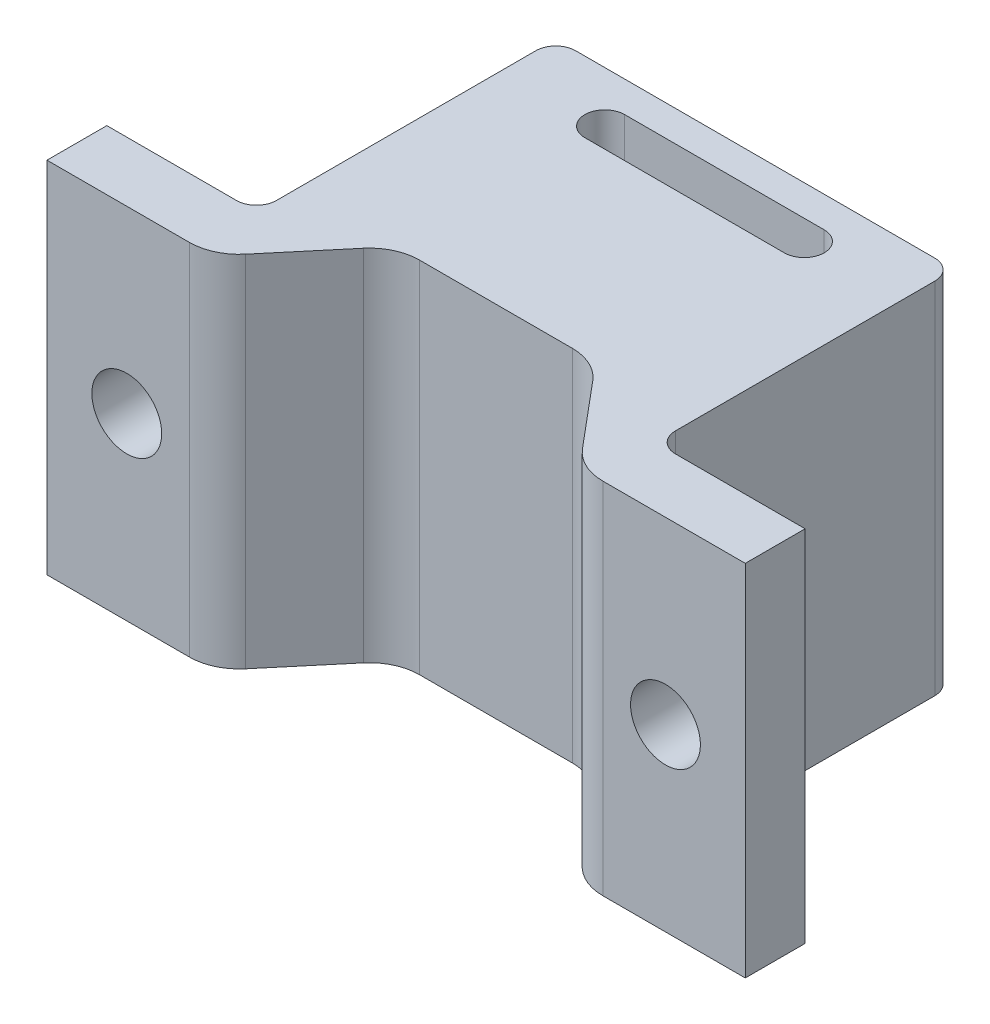
SolidWorks part; units mm, degrees
ref_plane "Front" through (0, 0, 0) normal (0, 0, 1) x (1, 0, 0)
ref_plane "Top" through (0, 0, 0) normal (0, 1, 0) x (1, 0, 0)
ref_plane "Right" through (0, 0, 0) normal (1, 0, 0) x (0, 0, -1)
sketch "Sketch1" plane through (0, 0, 0) normal (0, 1, 0) x (1, 0, 0)
  line L0 (-20, -13.7446) -> (-20, 16.2554)
  line L3 (-20, 16.2554) -> (20, 16.2554)
  line L5 (20, -13.7446) -> (20, 16.2554)
  line L6 (-18.391, -19.7446) -> (-10, -9.7446)
  line L7 (-35, -19.7446) -> (-18.391, -19.7446)
  line L8 (-35, -19.7446) -> (-35, -13.7446)
  line L9 (-35, -13.7446) -> (-20, -13.7446)
  line L10 (35, -19.7446) -> (35, -13.7446)
  line L11 (-10, -9.7446) -> (10, -9.7446)
  line L12 (10, -9.7446) -> (18.391, -19.7446)
  line L13 (20, -13.7446) -> (35, -13.7446)
  line L14 (18.391, -19.7446) -> (35, -19.7446)
  line L15 (-10, 11.1674) -> (10, 11.1674) construction
  line L16 (-10, 13.1674) -> (10, 13.1674)
  line L17 (-10, 9.1674) -> (10, 9.1674)
  arc A0 (-10, 13.1674) -> (-10, 9.1674) centre (-10, 11.1674) ccw
  arc A1 (10, 9.1674) -> (10, 13.1674) centre (10, 11.1674) ccw
  point P0 (0, 0)
  point P6 (0, -9.7446)
  point P11 (0, 11.1674)
  dimension "D14" = 2
  dimension "D1" = 70
  dimension "D2" = 36
  dimension "D3" = 40
  dimension "D4" = 15
  dimension "D5" = 20
  dimension "D6" = 6
  dimension "D7" = 6
  dimension "D8" = 0
  dimension "D9" = 20
  dimension "D10" = 10
  dimension "D11" = 80
  dimension "D12" = 40
  dimension "D13" = 40
extrude "Boss-Extrude1" add sketch "Sketch1" along normal blind 36
fillet "Fillet1" radius 5 4 edges at (18.391, 18, 19.7446) (10, 18, 9.7446) (-10, 18, 9.7446) (-18.391, 18, 19.7446)
fillet "Fillet2" radius 2 2 edges at (20, 18, 13.7446) (-20, 18, 13.7446)
sketch "Sketch2" plane through (0, 0, 13.7446) normal (0, 0, -1) x (-1, 0, 0)
  circle A0 centre (-27, 18) radius 3.5
  circle A1 centre (27, 18) radius 3.5
  dimension "D1" = 54
  dimension "D2" = 7
  dimension "D3" = 7
  dimension "D4" = 27
extrude "Cut-Extrude1" cut sketch "Sketch2" against normal through all
sketch "Sketch3" plane through (0, 0, -16.2554) normal (0, 0, -1) x (-1, 0, 0)
  line L1 (-20, 0) -> (20, 0) construction
  circle A0 centre (0, 18) radius 10
  dimension "D1" = 20
  dimension "D2" = 18
extrude "Cut-Extrude2" cut sketch "Sketch3" against normal blind 6
sketch "Sketch4" plane through (0, 0, -9.1674) normal (0, 0, -1) x (-1, 0, 0)
  circle A0 centre (0, 18) radius 8
  dimension "D1" = 16
extrude "Boss-Extrude2" add sketch "Sketch4" along normal blind 11.09
hole_wizard "M8 Tapped Hole1" positions "Sketch5" profile "Sketch6" tap size "M8" standard "GB"
sketch "Sketch5" plane through (0, 0, -20.2574) normal (0, 0, -1) x (-1, 0, 0)
  point P0 (0, 18)
sketch "Sketch6" plane through (0, 18, -20.2574) normal (1, 0, 0) x (0, 1, 0)
  line L0 (0, 0) -> (0, 24.2929)
  line L1 (0, 24.2929) -> (3.4, 22.25)
  line L2 (3.4, 22.25) -> (3.4, 0)
  line L5 (3.4, 0) -> (0, 0)
  line L10 (0, 24.2929) -> (-3.4, 22.25) construction
  line L11 (0, -6.35) -> (0, 107.95) construction
  dimension "螺纹孔钻头直径" = 6.8
  dimension "螺纹孔钻头深度" = 22.25
  dimension "导头角度" = 118
cosmetic thread "Tapped hole thread1" parameters "D1"=16, "D2"=8
fillet "Fillet3" radius 2 2 edges at (-20, 18, -16.2554) (20, 18, -16.2554)
